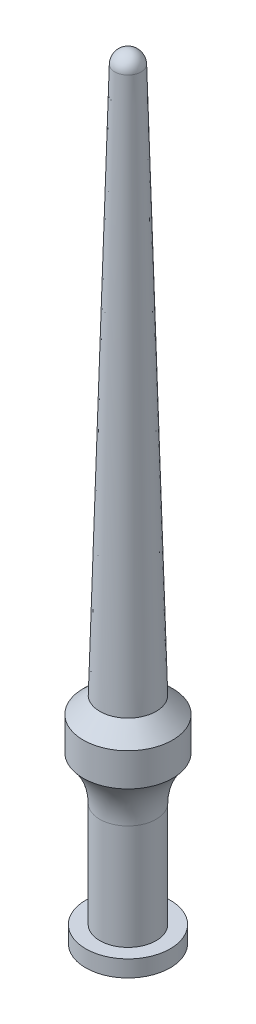
from build123d import *


with BuildPart() as part:
    # Sketch1 → Revolve1 (revolve)
    with BuildSketch(Plane.XY, mode=Mode.PRIVATE) as revolve1_sk:
        with BuildLine():
            Line((0, 0), (25.5, 0))
            Line((25.5, 0), (25.5, 10))
            Line((25.5, 10), (17, 10))
            Line((17, 10), (17, 73.542486889))
            ThreePointArc((17, 73.542486889), (19.583426132, 87.684622513), (27, 100))
            Line((27, 100), (27, 120))
            Line((27, 120), (17, 130))
            Line((17, 130), (7.997028415, 460.218028737))
            ThreePointArc((7.997028415, 460.218028737), (5.57923696, 465.733420876), (0, 468))
            Line((0, 468), (0, 0))
        make_face()
    revolve(revolve1_sk.sketch.rotate(Axis((0, 0, 0), (0, -1, 0)), 90), axis=Axis((0, 0, 0), (0, -1, 0)))


solid = part.part
